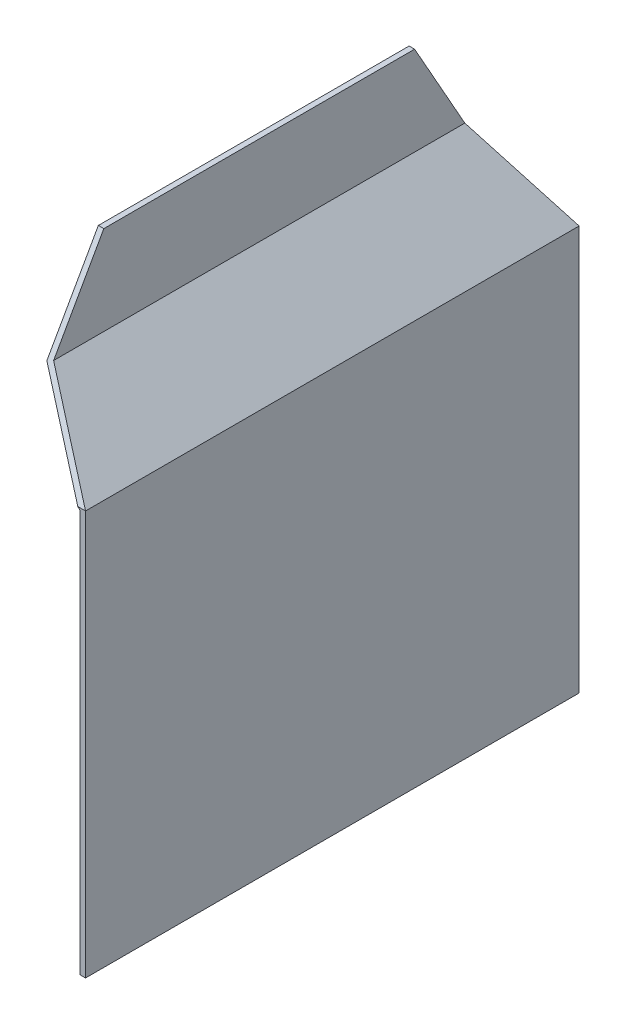
from build123d import *

# Parameters (mm, degrees)
EXTRUDE_1_DEPTH     = 270
CUT_EXTRUDE_2_DEPTH = 270


with BuildPart() as part:
    # 草图1 → 凸台-拉伸1 (new body)
    with BuildSketch(Plane.XY):
        Polygon((0, 0), (0, -50), (40, -90), (40, -310), (43, -310), (43, -88.757359313), (3, -48.757359313), (3, 0), align=None)
    extrude(amount=EXTRUDE_1_DEPTH)

    # 草图2 → 切除-拉伸2 (cut)
    with BuildSketch(Plane(origin=(43, 0, 0), x_dir=(0, 0, -1), z_dir=(1, 0, 0))):
        Polygon((-270, 0), (-220, 0), (-270, -88.757359313), align=None)
        Polygon((0, 0), (-50, 0), (0, -88.757359313), align=None)
    extrude(amount=-CUT_EXTRUDE_2_DEPTH, mode=Mode.SUBTRACT)


solid = part.part
